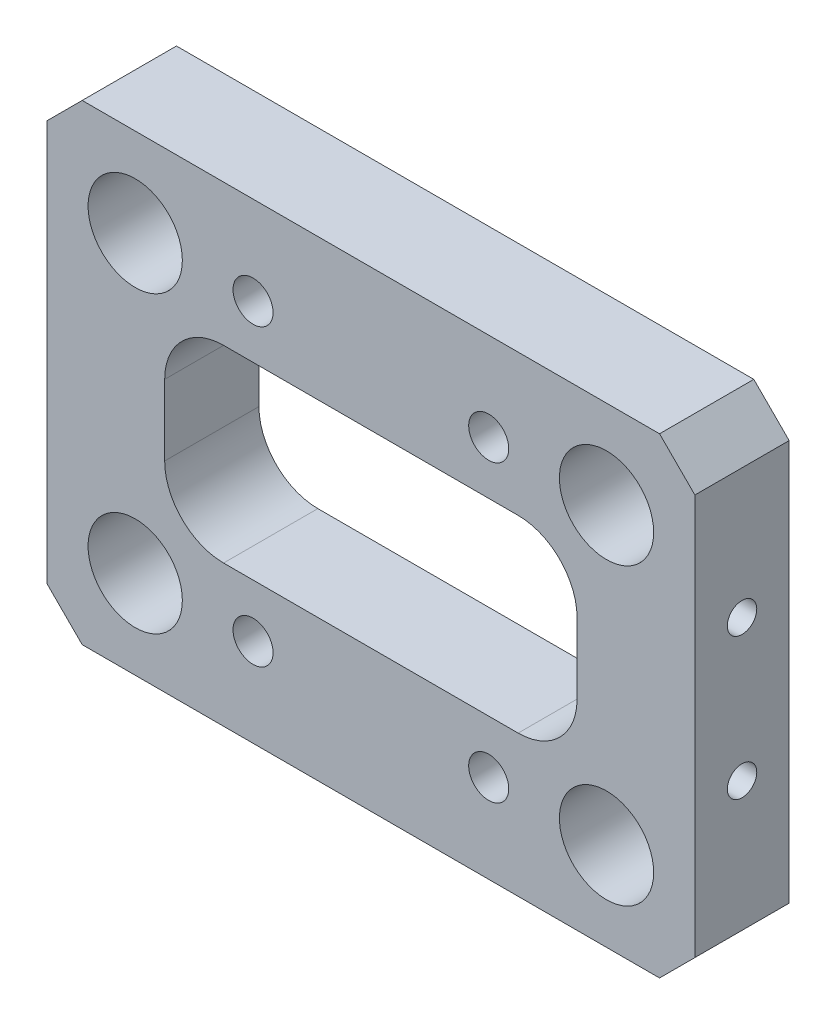
from build123d import *

# Parameters (mm, degrees)
SKETCH_1_W                   = 55
SKETCH_1_H                   = 40
EXTRUDE_1_DEPTH              = 8
SKETCH_2_W                   = 35
SKETCH_2_H                   = 16
CUT_EXTRUDE_1_DEPTH          = 35.932076949
HOLE_WIZARD_M3_1_D           = 3.4
HOLE_WIZARD_M3_1_CBORE_D     = 6
HOLE_WIZARD_M3_1_CBORE_DEPTH = 3.4
HOLE_WIZARD_M3_1_2_D         = 2.5
HOLE_WIZARD_M3_1_2_DEPTH     = 7.5
HOLE_WIZARD_M3_1_2_TIP       = 0.751075774
M8X1_0_1_D                   = 5
M8X1_0_1_CBORE_D             = 8
M8X1_0_1_CBORE_DEPTH         = 6
HOLE_WIZARD_M3_2_D           = 2.5
HOLE_WIZARD_M3_2_DEPTH       = 8.5
HOLE_WIZARD_M3_2_TIP         = 0.751075774
CHAMFER_1_SIZE               = 3
FILLET_1_R                   = 5


with BuildPart() as part:
    # 草图1 → 凸台-拉伸1 (new body)
    with BuildSketch(Plane.XY.offset(4)):
        Rectangle(SKETCH_1_W, SKETCH_1_H)
    extrude(amount=-EXTRUDE_1_DEPTH)

    # 草图2 → 切除-拉伸1 (cut, through all)
    with BuildSketch(Plane(origin=(0, 0, -4), x_dir=(-1, 0, 0), z_dir=(0, 0, -1))):
        Rectangle(SKETCH_2_W, SKETCH_2_H)
    extrude(amount=-CUT_EXTRUDE_1_DEPTH, mode=Mode.SUBTRACT)

    # Hole Wizard M3 _1 (through all)
    with Locations(Plane(origin=(0, 0, -4), x_dir=(-1, 0, 0), z_dir=(0, 0, -1))):
        with Locations((10, -12.5), (-10, -12.5), (10, 12.5), (-10, 12.5)):
            CounterBoreHole(HOLE_WIZARD_M3_1_D / 2, HOLE_WIZARD_M3_1_CBORE_D / 2, HOLE_WIZARD_M3_1_CBORE_DEPTH)

    # Hole Wizard M3 _1 2
    with Locations(Plane(origin=(27.5, 0, 0), x_dir=(0, 0, -1), z_dir=(1, 0, 0))):
        with Locations((0, 6), (0, -6)):
            Hole(HOLE_WIZARD_M3_1_2_D / 2, depth=HOLE_WIZARD_M3_1_2_DEPTH)
            with Locations((0, 0, -(HOLE_WIZARD_M3_1_2_DEPTH + HOLE_WIZARD_M3_1_2_TIP / 2))):  # 118° drill point
                Cone(0, HOLE_WIZARD_M3_1_2_D / 2, HOLE_WIZARD_M3_1_2_TIP, mode=Mode.SUBTRACT)

    # M8x1.0 螺纹孔1 (through all)
    with Locations(Plane.XY.offset(4)):
        with Locations((-20, 12.5), (-20, -12.5), (20, 12.5), (20, -12.5)):
            CounterBoreHole(M8X1_0_1_D / 2, M8X1_0_1_CBORE_D / 2, M8X1_0_1_CBORE_DEPTH)

    # M3 螺纹孔2
    with Locations(Plane.ZY.offset(27.5)):
        with Locations((0, 6), (0, -6)):
            Hole(HOLE_WIZARD_M3_2_D / 2, depth=HOLE_WIZARD_M3_2_DEPTH)
            with Locations((0, 0, -(HOLE_WIZARD_M3_2_DEPTH + HOLE_WIZARD_M3_2_TIP / 2))):  # 118° drill point
                Cone(0, HOLE_WIZARD_M3_2_D / 2, HOLE_WIZARD_M3_2_TIP, mode=Mode.SUBTRACT)

    # 倒角1
    chamfer_1_edges = [part.edges().sort_by_distance(p)[0] for p in [
        (27.5, 20, 0),
        (27.5, -20, 0),
        (-27.5, -20, 0),
        (-27.5, 20, 0),
    ]]
    chamfer(chamfer_1_edges, length=CHAMFER_1_SIZE)

    # 圆角1
    fillet_1_edges = [part.edges().sort_by_distance(p)[0] for p in [
        (-17.5, -8, 0),
        (17.5, -8, 0),
        (17.5, 8, 0),
        (-17.5, 8, 0),
    ]]
    fillet(fillet_1_edges, radius=FILLET_1_R)


solid = part.part
